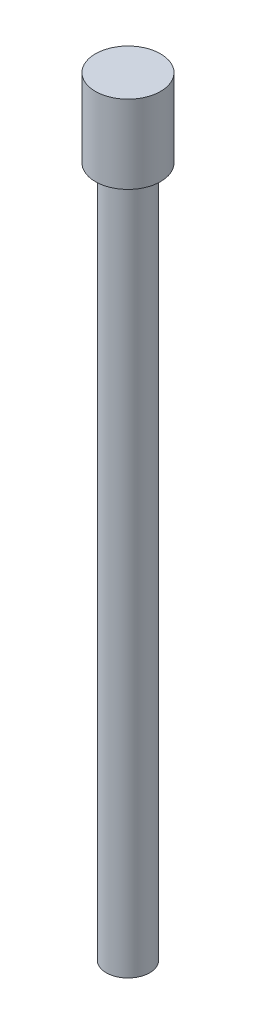
from build123d import *


with BuildPart() as part:
    # Sketch1 → Revolve1 (revolve)
    with BuildSketch(Plane.XY, mode=Mode.PRIVATE) as revolve1_sk:
        Polygon((0, 0), (20, 0), (20, 636), (30, 636), (30, 708), (0, 708), align=None)
    revolve(revolve1_sk.sketch.rotate(Axis((0, 0, 0), (0, -1, 0)), 90), axis=Axis((0, 0, 0), (0, -1, 0)))


solid = part.part
